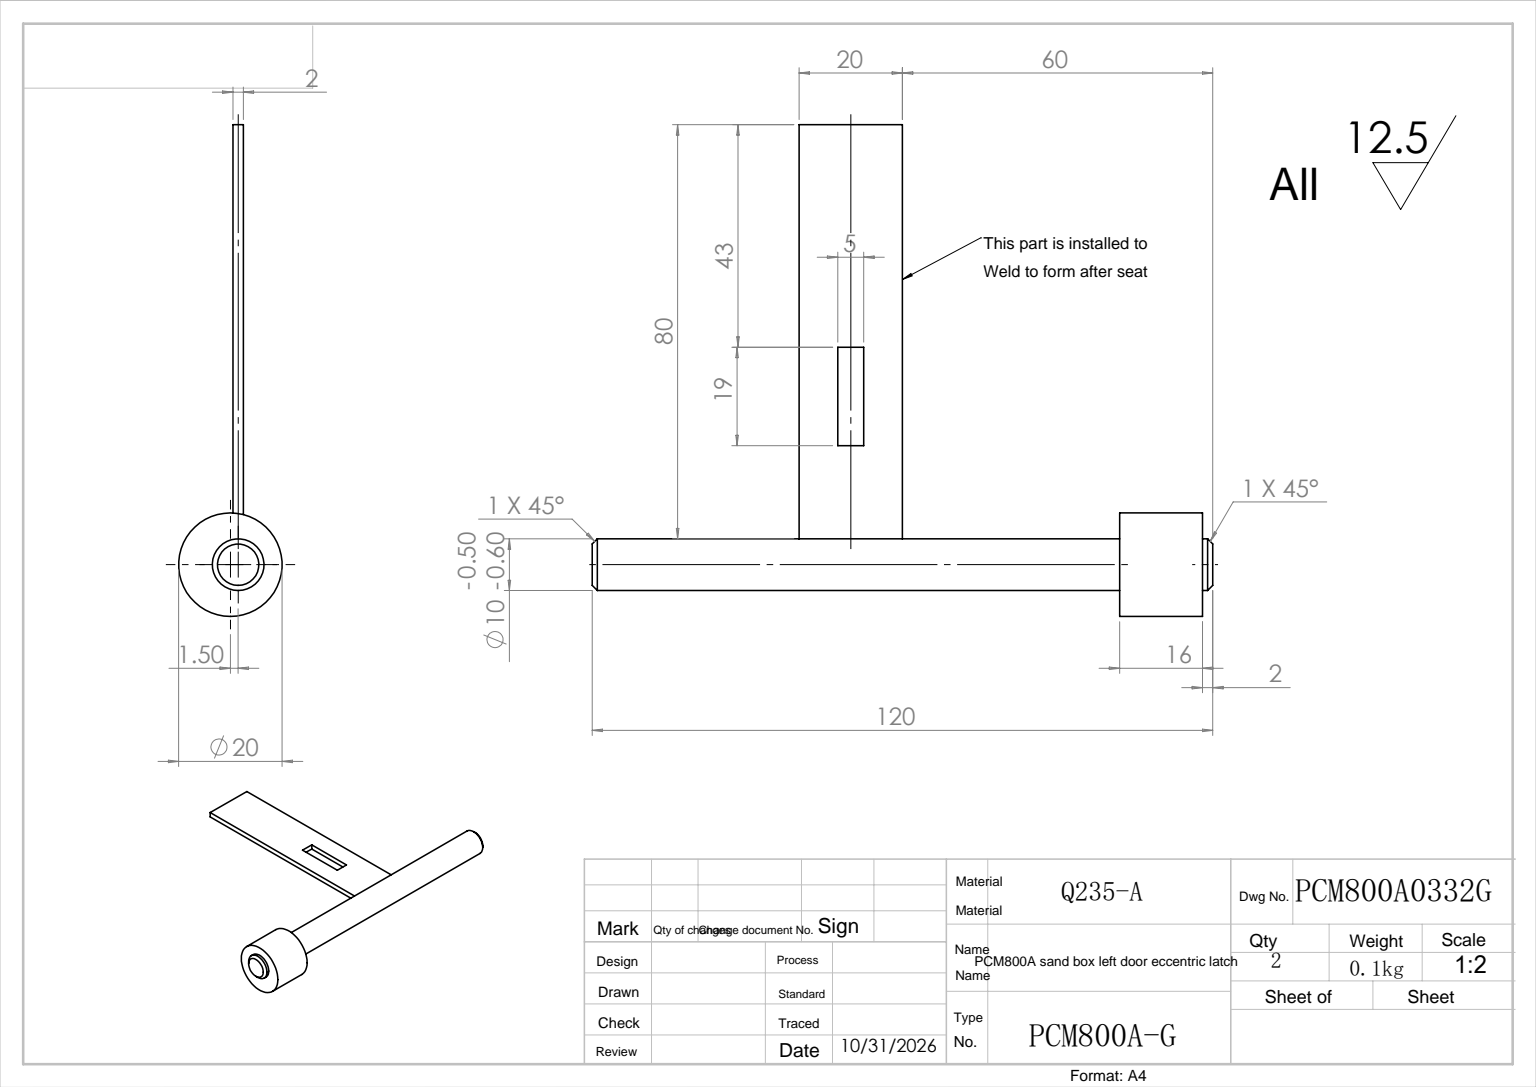
SolidWorks part; units mm, degrees
ref_plane "前视基准面" through (0, 0, 0) normal (0, 0, 1) x (1, 0, 0)
ref_plane "上视基准面" through (0, 0, 0) normal (0, 1, 0) x (1, 0, 0)
ref_plane "右视基准面" through (0, 0, 0) normal (1, 0, 0) x (0, 0, -1)
sketch "草图1" plane through (0, 0, 0) normal (0, 0, 1) x (1, 0, 0)
  circle A0 centre (0, 0) radius 5
  dimension "D1" = 10
extrude "凸台-拉伸1" add sketch "草图1" along normal blind 120
sketch "草图2" plane through (0, 0, 120) normal (0, 0, 1) x (1, 0, 0)
  circle A0 centre (0, -1.5) radius 10
  circle A1 centre (0, 0) radius 5 construction
  dimension "D1" = 1.5
  dimension "D2" = 20
extrude "凸台-拉伸2" add sketch "草图2" against normal blind 16 from offset 2 offset against normal yes
sketch "草图3" plane through (0, 0, 0) normal (0, 1, 0) x (1, 0, 0)
  line L0 (-5, 0) -> (-5, -102) construction
  line L1 (-5, -40) -> (-85, -40)
  line L2 (-5, -40) -> (-5, -60)
  line L3 (-5, -60) -> (-85, -60)
  line L4 (-85, -40) -> (-85, -60)
  line L5 (-5, -120) -> (5, -120) construction
  line L7 (-42, -47.5) -> (-23, -47.5)
  line L8 (-42, -47.5) -> (-42, -52.5)
  line L9 (-42, -52.5) -> (-23, -52.5)
  line L10 (-23, -47.5) -> (-23, -52.5)
  dimension "D1" = 80
  dimension "D2" = 20
  dimension "D3" = 60
  dimension "D4" = 5
  dimension "D5" = 19
  dimension "D6" = 43
  dimension "D7" = 7.5
extrude "凸台-拉伸3" add sketch "草图3" along normal mid plane 2 separate body
chamfer "倒角1" distance 1 angle 45 2 edges at (5, 0, 120) (5, 0, 0)
